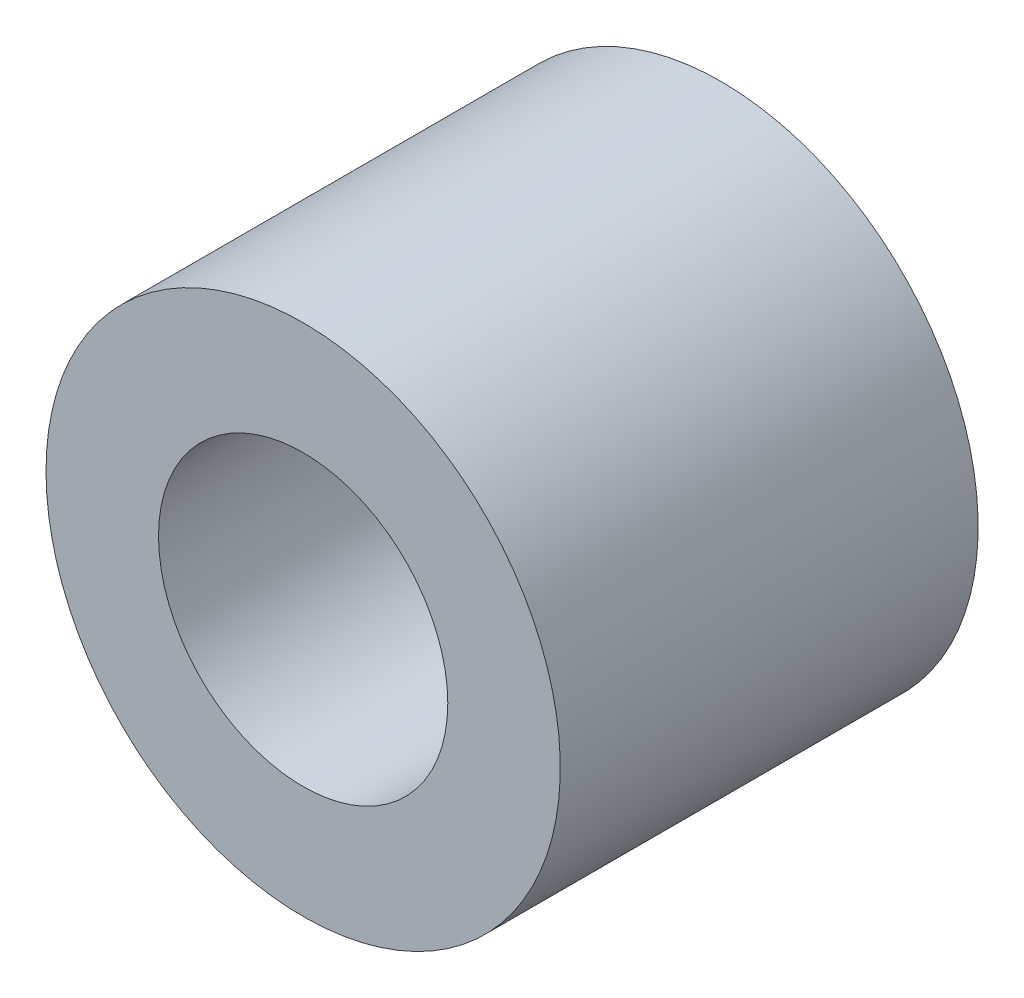
from build123d import *

# Parameters (mm, degrees)
SKETCH_4_R          = 4
EXTRUDE_1_DEPTH     = 6.5
SKETCH_9_R          = 2.25
CUT_EXTRUDE_1_DEPTH = 9.61684397


with BuildPart() as part:
    # 草图4 → 凸台-拉伸1 (new body)
    with BuildSketch(Plane.XY):
        with Locations(Location((0, 0, 0), (0, 0, 180))):
            Circle(SKETCH_4_R)
    extrude(amount=EXTRUDE_1_DEPTH)

    # 草图9 → 切除-拉伸1 (cut, through all)
    with BuildSketch(Plane.XY.offset(6.5)):
        Circle(SKETCH_9_R)
    extrude(amount=-CUT_EXTRUDE_1_DEPTH, mode=Mode.SUBTRACT)


solid = part.part
